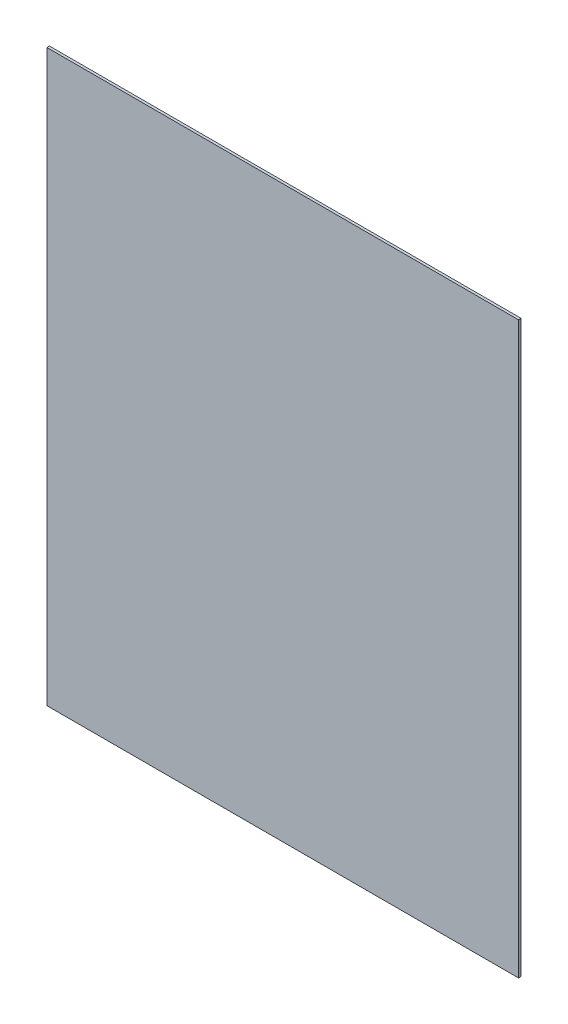
from build123d import *

# Parameters (mm, degrees)
SKETCH_1_W      = 926
SKETCH_1_H      = 1119
EXTRUDE_1_DEPTH = 5


with BuildPart() as part:
    # 草图1 → 凸台-拉伸1 (new body)
    with BuildSketch(Plane.XY):
        Rectangle(SKETCH_1_W, SKETCH_1_H)
    extrude(amount=EXTRUDE_1_DEPTH)


solid = part.part
